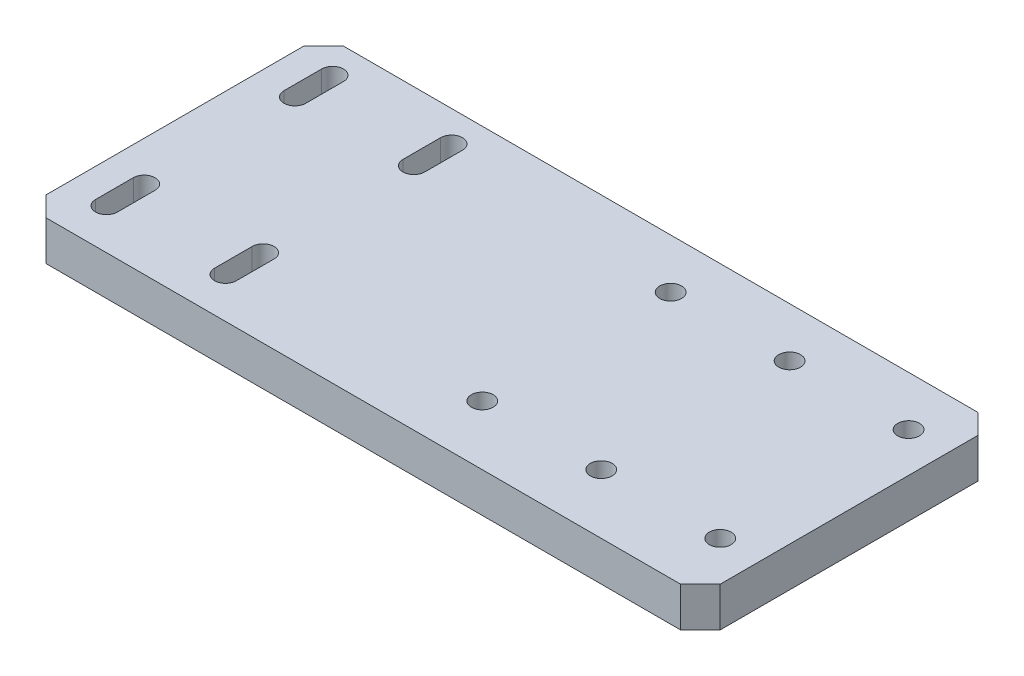
SolidWorks part; units mm, degrees
material "A6061 T6"
ref_plane "前视基准面" through (0, 0, 0) normal (0, 0, 1) x (1, 0, 0)
ref_plane "上视基准面" through (0, 0, 0) normal (0, 1, 0) x (1, 0, 0)
ref_plane "右视基准面" through (0, 0, 0) normal (1, 0, 0) x (0, 0, -1)
sketch "草图1" plane through (0, 0, 0) normal (0, 1, 0) x (1, 0, 0)
  line L1 (-85, 37.5) -> (85, 37.5)
  line L2 (-85, 37.5) -> (-85, -37.5)
  line L3 (-85, -37.5) -> (85, -37.5)
  line L4 (85, 37.5) -> (85, -37.5)
  line L5 (-85, 37.5) -> (85, -37.5) construction
  line L6 (-85, -37.5) -> (85, 37.5) construction
  point P0 (0, 0)
  dimension "D1" = 170
  dimension "D2" = 75
extrude "凸台-拉伸1" add sketch "草图1" along normal blind 10
chamfer "倒角1" distance 5 angle 45 4 edges at (-85, 5, -37.5) (85, 5, -37.5) (85, 5, 37.5) (-85, 5, 37.5)
sketch "草图2" plane through (0, 10, 0) normal (0, 1, 0) x (1, 0, 0)
  line L0 (-75, 29.75) -> (-75, 20.25) construction
  line L1 (-72.25, 29.75) -> (-72.25, 20.25)
  line L2 (-77.75, 29.75) -> (-77.75, 20.25)
  line L3 (-45, 29.75) -> (-45, 20.25) construction
  line L4 (-42.25, 29.75) -> (-42.25, 20.25)
  line L5 (-47.75, 29.75) -> (-47.75, 20.25)
  line L6 (-75, -17.75) -> (-75, -27.25) construction
  line L7 (-72.25, -17.75) -> (-72.25, -27.25)
  line L8 (-77.75, -17.75) -> (-77.75, -27.25)
  line L9 (-45, -17.75) -> (-45, -27.25) construction
  line L10 (-42.25, -17.75) -> (-42.25, -27.25)
  line L11 (-47.75, -17.75) -> (-47.75, -27.25)
  circle A0 centre (15, 25) radius 2.75
  circle A1 centre (45, 25) radius 2.75
  circle A2 centre (75, 25) radius 2.75
  circle A3 centre (15, -22.5) radius 2.75
  circle A4 centre (45, -22.5) radius 2.75
  circle A5 centre (75, -22.5) radius 2.75
  arc A6 (-72.25, 29.75) -> (-77.75, 29.75) centre (-75, 29.75) ccw
  arc A7 (-77.75, 20.25) -> (-72.25, 20.25) centre (-75, 20.25) ccw
  arc A8 (-42.25, 29.75) -> (-47.75, 29.75) centre (-45, 29.75) ccw
  arc A9 (-47.75, 20.25) -> (-42.25, 20.25) centre (-45, 20.25) ccw
  arc A10 (-72.25, -17.75) -> (-77.75, -17.75) centre (-75, -17.75) ccw
  arc A11 (-77.75, -27.25) -> (-72.25, -27.25) centre (-75, -27.25) ccw
  arc A12 (-42.25, -17.75) -> (-47.75, -17.75) centre (-45, -17.75) ccw
  arc A13 (-47.75, -27.25) -> (-42.25, -27.25) centre (-45, -27.25) ccw
  point P22 (-75, 25)
  point P27 (-45, 25)
  point P36 (-75, -22.5)
  point P45 (-45, -22.5)
  dimension "D1" = 5.5
  dimension "D2" = 2.75
extrude "切除-拉伸1" cut sketch "草图2" against normal blind 15
